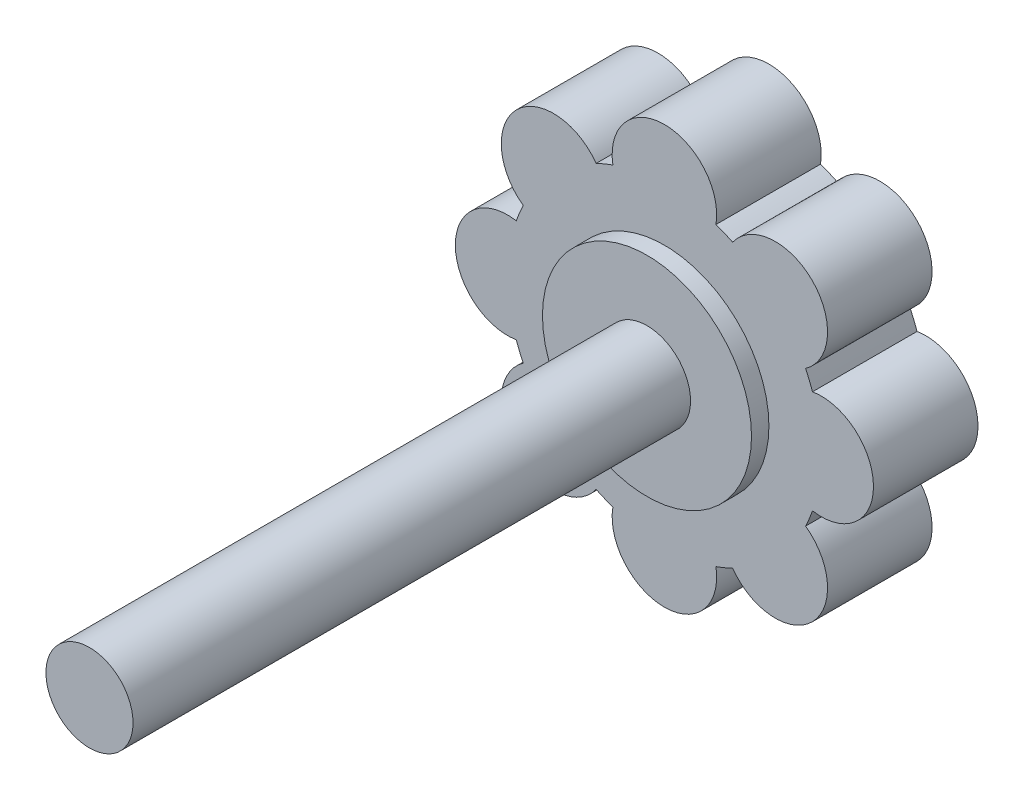
from build123d import *

# Parameters (mm, degrees)
BOSS_EXTRUDE1_DEPTH = 6
SKETCH2_R           = 2.5
BOSS_EXTRUDE2_DEPTH = 33
SKETCH3_R           = 6
BOSS_EXTRUDE3_DEPTH = 1
SKETCH4_R           = 3.704648002
CUT_EXTRUDE1_DEPTH  = 0.2


with BuildPart() as part:
    # Sketch1 → Boss-Extrude1 (new body)
    with BuildSketch(Plane.XY):
        with BuildLine():
            ThreePointArc((-8.5, -2.958039892), (-8.314915793, -3.444150891), (-8.102057706, -3.918757574))
            ThreePointArc((-8.102057706, -3.918757574), (-8.485281374, -8.485281374), (-3.918757574, -8.102057706))
            ThreePointArc((-3.918757574, -8.102057706), (-3.444150891, -8.314915793), (-2.958039892, -8.5))
            ThreePointArc((-2.958039892, -8.5), (0, -12), (2.958039892, -8.5))
            ThreePointArc((2.958039892, -8.5), (3.444150891, -8.314915793), (3.918757574, -8.102057706))
            ThreePointArc((3.918757574, -8.102057706), (8.485281374, -8.485281374), (8.102057706, -3.918757574))
            ThreePointArc((8.102057706, -3.918757574), (8.314915793, -3.444150891), (8.5, -2.958039892))
            ThreePointArc((8.5, -2.958039892), (12, 0), (8.5, 2.958039892))
            ThreePointArc((8.5, 2.958039892), (8.314915793, 3.444150891), (8.102057706, 3.918757574))
            ThreePointArc((8.102057706, 3.918757574), (8.485281374, 8.485281374), (3.918757574, 8.102057706))
            ThreePointArc((3.918757574, 8.102057706), (3.444150891, 8.314915793), (2.958039892, 8.5))
            ThreePointArc((2.958039892, 8.5), (0, 12), (-2.958039892, 8.5))
            ThreePointArc((-2.958039892, 8.5), (-3.444150891, 8.314915793), (-3.918757574, 8.102057706))
            ThreePointArc((-3.918757574, 8.102057706), (-8.485281374, 8.485281374), (-8.102057706, 3.918757574))
            ThreePointArc((-8.102057706, 3.918757574), (-8.314915793, 3.444150891), (-8.5, 2.958039892))
            ThreePointArc((-8.5, 2.958039892), (-12, 0), (-8.5, -2.958039892))
        make_face()
    extrude(amount=BOSS_EXTRUDE1_DEPTH)

    # Sketch2 → Boss-Extrude2 (add)
    with BuildSketch(Plane.XY.offset(6)):
        Circle(SKETCH2_R)
    extrude(amount=BOSS_EXTRUDE2_DEPTH)

    # Sketch3 → Boss-Extrude3 (add, symmetric)
    with BuildSketch(Plane.XY.offset(6)):
        Circle(SKETCH3_R)
    extrude(amount=BOSS_EXTRUDE3_DEPTH, both=True)

    # Sketch4 → Cut-Extrude1 (cut)
    with BuildSketch(Plane(origin=(0, 0, 0), x_dir=(-1, 0, 0), z_dir=(0, 0, -1))):
        Circle(SKETCH4_R)
    extrude(amount=-CUT_EXTRUDE1_DEPTH, mode=Mode.SUBTRACT)


solid = part.part
